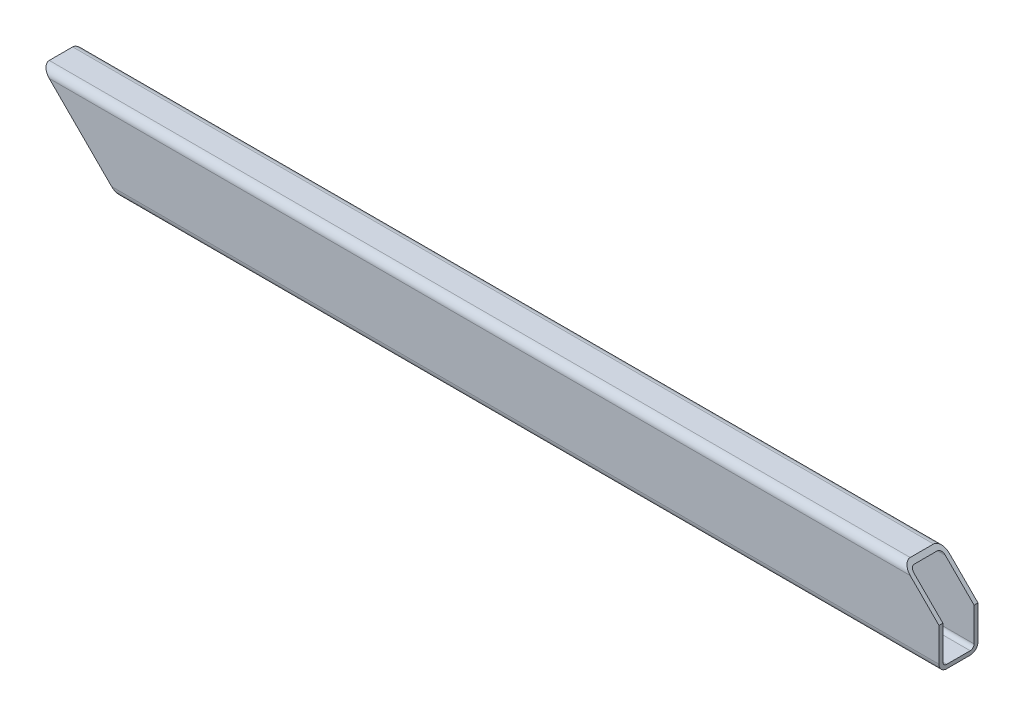
from build123d import *

# Parameters (mm, degrees)
F_100_X_50_X_5_1_DEPTH = 1150
CUT_EXTRUDE_1_REACH    = 1159.854


with BuildPart() as part:
    # Sketch11 → 矩形管 100 X 50 X 5(1) (new body)
    with BuildSketch(Plane(origin=(0, 0, 0), x_dir=(0, 0, -1), z_dir=(1, 0, 0))):
        with BuildLine():
            Line((-15, -50), (15, -50))
            ThreePointArc((15, -50), (22.071067812, -47.071067812), (25, -40))
            Line((25, -40), (25, 40))
            ThreePointArc((25, 40), (22.071067812, 47.071067812), (15, 50))
            Line((15, 50), (-15, 50))
            ThreePointArc((-15, 50), (-22.071067812, 47.071067812), (-25, 40))
            Line((-25, 40), (-25, -40))
            ThreePointArc((-25, -40), (-22.071067812, -47.071067812), (-15, -50))
        make_face()
        with BuildLine():
            Line((-15, -45), (15, -45))
            ThreePointArc((15, -45), (18.535533906, -43.535533906), (20, -40))
            Line((20, -40), (20, 40))
            ThreePointArc((20, 40), (18.535533906, 43.535533906), (15, 45))
            Line((15, 45), (-15, 45))
            ThreePointArc((-15, 45), (-18.535533906, 43.535533906), (-20, 40))
            Line((-20, 40), (-20, -40))
            ThreePointArc((-20, -40), (-18.535533906, -43.535533906), (-15, -45))
        make_face(mode=Mode.SUBTRACT)
    extrude(amount=F_100_X_50_X_5_1_DEPTH)

    # 切除-拉伸1: up to this face of the body (flat: up to its plane)
    cut_extrude_1_end = Plane(part.part.faces().sort_by_distance((575, 0, -25))[0])
    # 草图2 → 切除-拉伸1 (cut, up to the picked face)
    with BuildSketch(Plane(origin=(0, 75, 25), x_dir=(1, 0, 0), z_dir=(0, 0, 1)), mode=Mode.PRIVATE) as cut_extrude_1_sk1:
        Polygon((0, -25), (100, -125), (0, -125), align=None)
    cut_extrude_1_tool1 = split(extrude(cut_extrude_1_sk1.sketch, amount=-CUT_EXTRUDE_1_REACH, mode=Mode.PRIVATE), bisect_by=cut_extrude_1_end, keep=Keep.BOTH, mode=Mode.PRIVATE)
    # 草图2 → 切除-拉伸1 (cut, up to the picked face)
    with BuildSketch(Plane(origin=(0, 75, 25), x_dir=(1, 0, 0), z_dir=(0, 0, 1)), mode=Mode.PRIVATE) as cut_extrude_1_sk2:
        Polygon((1150, -71.913421349), (1103.086578651, -25), (1150, -25), align=None)
    cut_extrude_1_tool2 = split(extrude(cut_extrude_1_sk2.sketch, amount=-CUT_EXTRUDE_1_REACH, mode=Mode.PRIVATE), bisect_by=cut_extrude_1_end, keep=Keep.BOTH, mode=Mode.PRIVATE)
    add(cut_extrude_1_tool1.solids().sort_by(Axis((33.333333, -16.666667, 25), (0, 0, -1)))[0], mode=Mode.SUBTRACT)
    add(cut_extrude_1_tool2.solids().sort_by(Axis((1134.362193, 34.362193, 25), (0, 0, -1)))[0], mode=Mode.SUBTRACT)


solid = part.part
